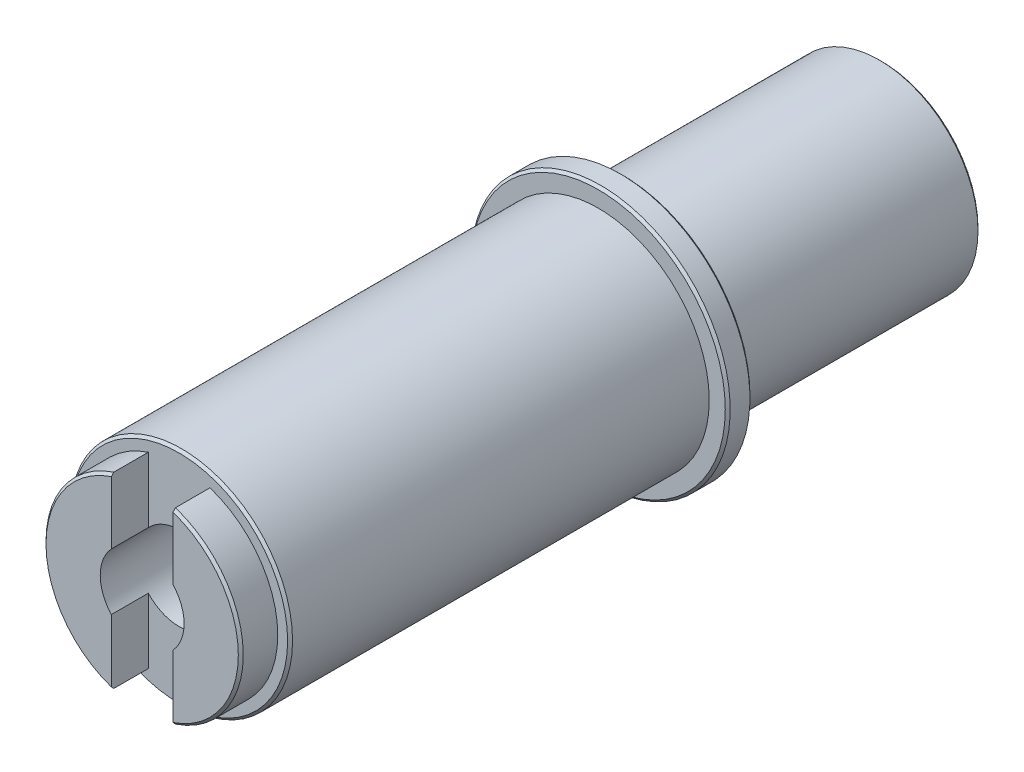
SolidWorks part; units mm, degrees
ref_plane "前视基准面" through (0, 0, 0) normal (0, 0, 1) x (1, 0, 0)
ref_plane "上视基准面" through (0, 0, 0) normal (0, 1, 0) x (1, 0, 0)
ref_plane "右视基准面" through (0, 0, 0) normal (1, 0, 0) x (0, 0, -1)
sketch "草图1" plane through (0, 0, 0) normal (0, 0, 1) x (1, 0, 0)
  circle A0 centre (0, 0) radius 9
  dimension "D1" = 18
extrude "凸台-拉伸1" add sketch "草图1" along normal blind 34
sketch "草图2" plane through (0, 0, 34) normal (0, 0, 1) x (1, 0, 0)
  circle A0 centre (0, 0) radius 8
  dimension "D1" = 16
extrude "凸台-拉伸2" add sketch "草图2" along normal blind 3
sketch "草图3" plane through (0, 0, 0) normal (0, 0, -1) x (-1, 0, 0)
  circle A0 centre (0, 0) radius 10.5
  dimension "D1" = 21
extrude "凸台-拉伸3" add sketch "草图3" along normal blind 2
sketch "草图4" plane through (0, 0, -2) normal (0, 0, -1) x (-1, 0, 0)
  circle A0 centre (0, 0) radius 8
  dimension "D1" = 16
extrude "凸台-拉伸4" add sketch "草图4" along normal blind 21
sketch "草图5" plane through (0, 0, 37) normal (0, 0, 1) x (1, 0, 0)
  line L0 (0, 0) -> (0, 28.2926) construction
  line L1 (-2.5, -14.2936) -> (2.5, -14.2936)
  line L2 (-2.5, -14.2936) -> (-2.5, 18.1568)
  line L3 (-2.5, 18.1568) -> (2.5, 18.1568)
  line L4 (2.5, -14.2936) -> (2.5, 18.1568)
  dimension "D1" = 5
extrude "切除-拉伸1" cut sketch "草图5" against normal blind 3
hole_wizard "M8 螺纹孔1" positions "草图9" profile "草图7" tap size "M8" standard "GB"
sketch "草图9" plane through (0, 0, 37) normal (0, 0, 1) x (1, 0, 0)
  point P0 (0, 0)
sketch "草图7" plane through (0, 0, 37) normal (1, 0, 0) x (0, -1, 0)
  line L0 (0, 0) -> (0, 21.7929)
  line L1 (0, 21.7929) -> (3.4, 19.75)
  line L2 (3.4, 19.75) -> (3.4, 0)
  line L5 (3.4, 0) -> (0, 0)
  line L10 (0, 21.7929) -> (-3.4, 19.75) construction
  line L11 (0, -6.35) -> (0, 107.95) construction
  dimension "螺纹孔钻头直径" = 6.8
  dimension "螺纹孔钻头深度" = 19.75
  dimension "导头角度" = 118
cosmetic thread "孔螺蚊线1" parameters "D1"=16, "D2"=8
chamfer "倒角1" distance 0.2 angle 45 6 edges at (-8, 0, -23) (-10.5, 0, -2) (-10.5, 0, 0) (9, 0, 34) (8, 0, 37) (-8, 0, 37)
